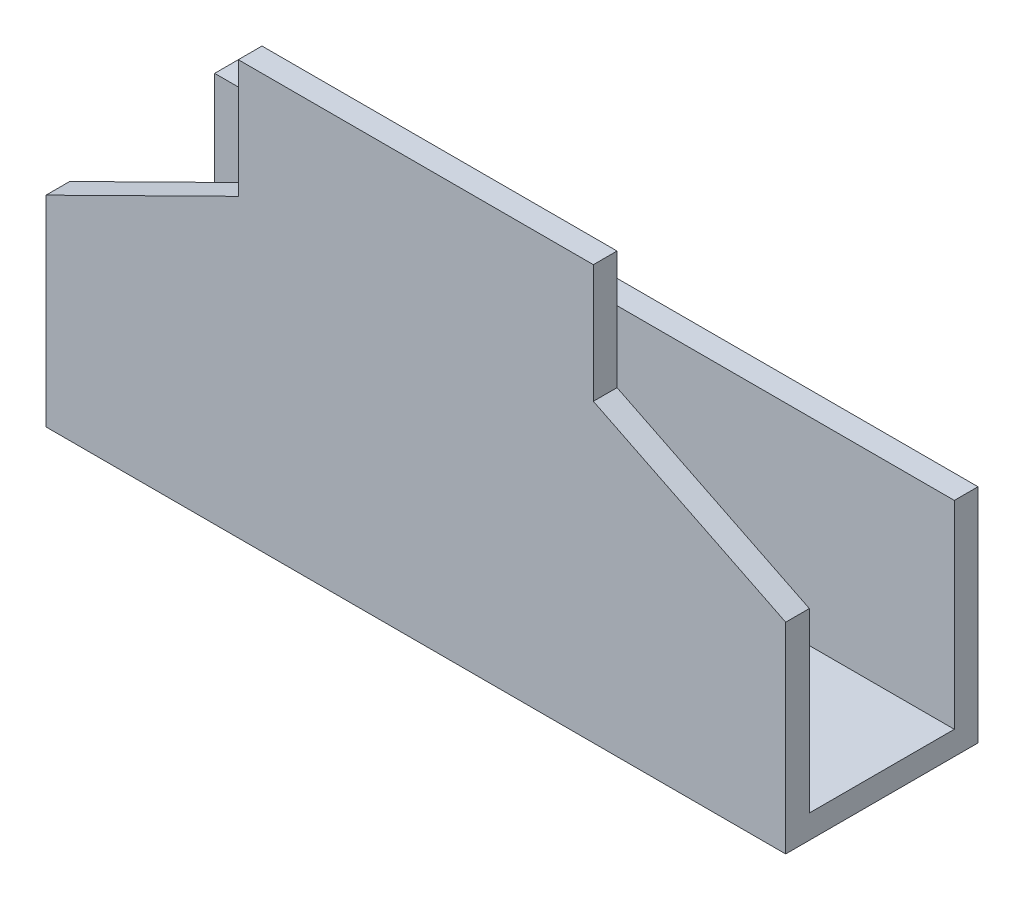
from build123d import *

# Parameters (mm, degrees)
BOSS_EXTRUDE1_DEPTH = 16
SKETCH2_W           = 500
SKETCH2_H           = 16
BOSS_EXTRUDE2_DEPTH = 130
SKETCH3_W           = 500
SKETCH3_H           = 16
BOSS_EXTRUDE3_DEPTH = 150


with BuildPart() as part:
    # Sketch1 → Boss-Extrude1 (new body)
    with BuildSketch(Plane.XY):
        Polygon((120, 280), (-120, 280), (-120, 200), (-250, 135.697802275), (-250, 0), (250, 0), (250, 135.697802275), (120, 200), align=None)
    extrude(amount=BOSS_EXTRUDE1_DEPTH)

    # Sketch2 → Boss-Extrude2 (add)
    with BuildSketch(Plane.XY.offset(16)):
        with Locations((0, 8)):
            Rectangle(SKETCH2_W, SKETCH2_H)
    extrude(amount=-BOSS_EXTRUDE2_DEPTH)

    # Sketch3 → Boss-Extrude3 (add)
    with BuildSketch(Plane(origin=(0, 0, 0), x_dir=(-1, 0, 0), z_dir=(0, -1, 0))):
        with Locations((0, 106)):
            Rectangle(SKETCH3_W, SKETCH3_H)
    extrude(amount=-BOSS_EXTRUDE3_DEPTH)


solid = part.part
